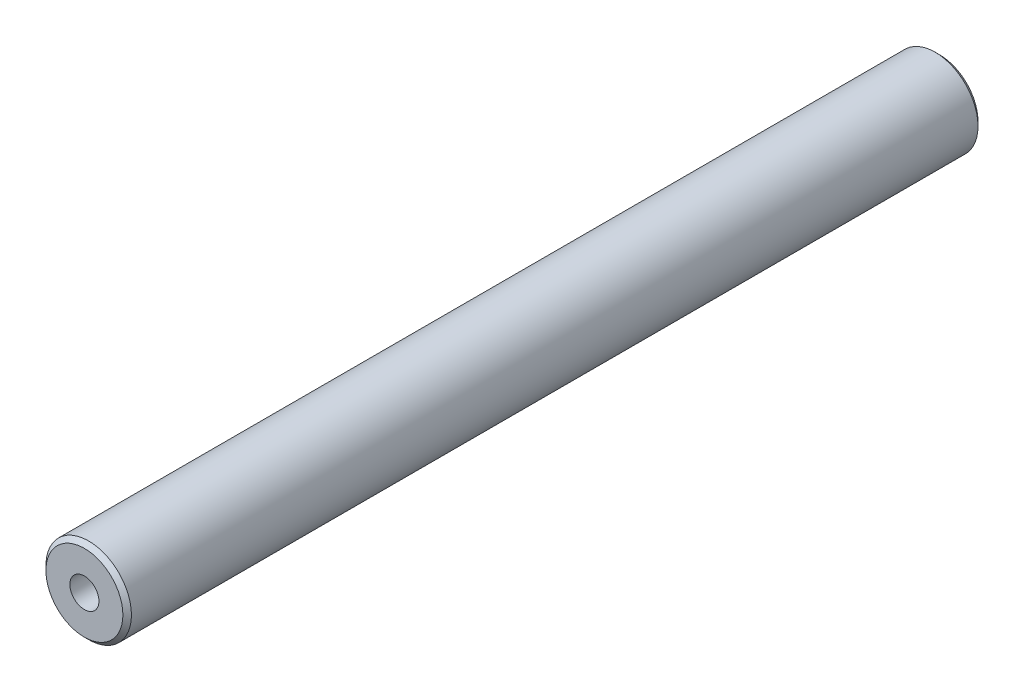
from build123d import *

# Parameters (mm, degrees)
SKETCH_1_R             = 10
EXTRUDE_1_DEPTH        = 200
HOLE_WIZARD_M8_1_D     = 6.8
HOLE_WIZARD_M8_1_DEPTH = 19.75
HOLE_WIZARD_M8_1_TIP   = 2.042926105
HOLE_WIZARD_M8_2_D     = 6.8
HOLE_WIZARD_M8_2_DEPTH = 19.75
HOLE_WIZARD_M8_2_TIP   = 2.042926105
CHAMFER_1_SIZE         = 1


with BuildPart() as part:
    # 草图1 → 凸台-拉伸1 (new body)
    with BuildSketch(Plane.XY):
        Circle(SKETCH_1_R)
    extrude(amount=EXTRUDE_1_DEPTH)

    # M8 螺纹孔1
    with Locations(Plane(origin=(0, 0, 0), x_dir=(-1, 0, 0), z_dir=(0, 0, -1))):
        with Locations((0, 0)):
            Hole(HOLE_WIZARD_M8_1_D / 2, depth=HOLE_WIZARD_M8_1_DEPTH)
            with Locations((0, 0, -(HOLE_WIZARD_M8_1_DEPTH + HOLE_WIZARD_M8_1_TIP / 2))):  # 118° drill point
                Cone(0, HOLE_WIZARD_M8_1_D / 2, HOLE_WIZARD_M8_1_TIP, mode=Mode.SUBTRACT)

    # M8 螺纹孔2
    with Locations(Plane.XY.offset(200)):
        with Locations((0, 0)):
            Hole(HOLE_WIZARD_M8_2_D / 2, depth=HOLE_WIZARD_M8_2_DEPTH)
            with Locations((0, 0, -(HOLE_WIZARD_M8_2_DEPTH + HOLE_WIZARD_M8_2_TIP / 2))):  # 118° drill point
                Cone(0, HOLE_WIZARD_M8_2_D / 2, HOLE_WIZARD_M8_2_TIP, mode=Mode.SUBTRACT)

    # 倒角1
    chamfer_1_edges = [part.edges().sort_by_distance(p)[0] for p in [
        (-10, 0, 0),
        (-10, 0, 200),
    ]]
    chamfer(chamfer_1_edges, length=CHAMFER_1_SIZE)


solid = part.part
